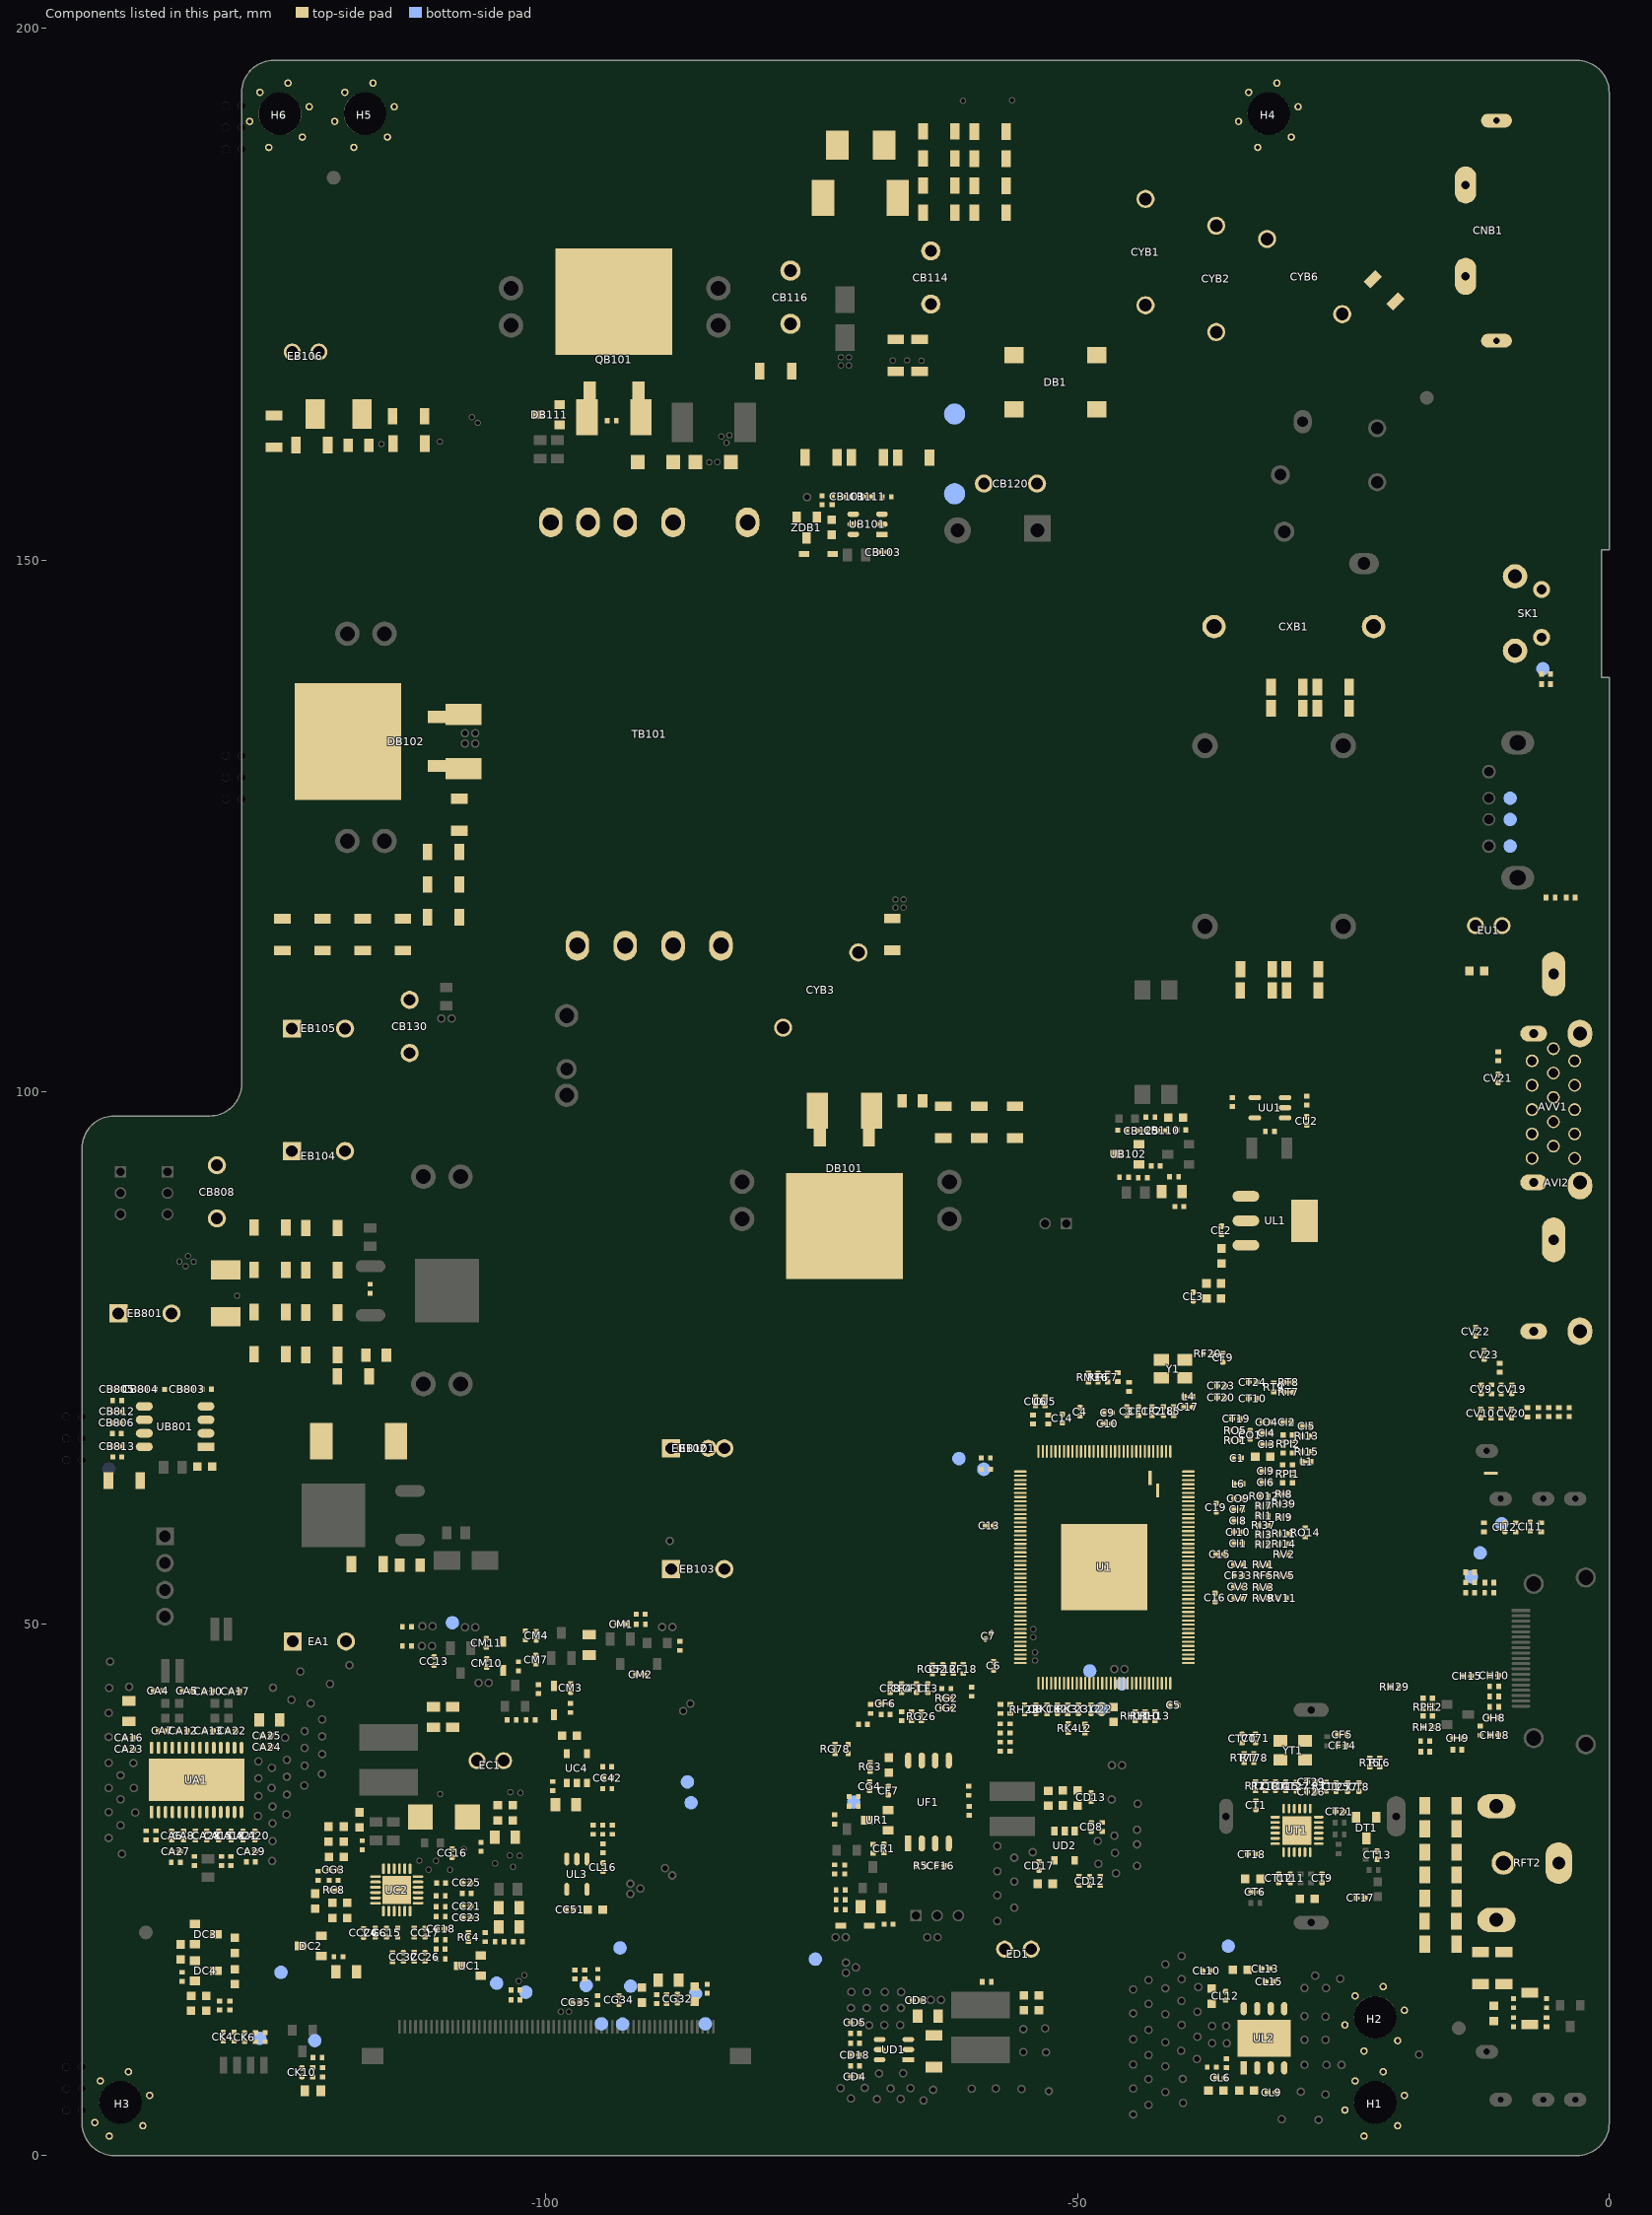
[diagram p0: the components of this part, seen from the top]
# Altium PCB MISC86383-9.PcbDoc (part 4 of 18)
Units mm, origin at the board's own origin, x right, y up, seen from the top; angles counter-clockwise.
Board outline 143.6 x 197 mm, 2 copper layers (TopLayer, BottomLayer), stack 1.571 mm thick; 743 components, 401 nets, 2996 pads, 1077 vias.
Unrouted connection lines stored in the file: 4.

## Components (designator, comment, footprint, x,y, rotation, side; value= is the part's Value field where it differs from the comment) (continued)
RH2 "Thick film resistor,RES,1/16W,0ohm,±1%,0402,SMD" R0402#1 -11.277,52.901 r0 top
RH10 "Thick film resistor,RES,1/16W,22ohm,±1%,0402,SMD" R0402#2 -43.635,41.317 r270 top
RH11 "Thick film resistor,RES,1/16W,22ohm,±1%,0402,SMD" R0402#2 -44.552,41.317 r270 top
RH13 "Thick film resistor,RES,1/16W,220ohm,±1%,0402,SMD" R0402#2 -42.714,41.317 r90 top
RH14 "Thick film resistor,RES,1/16W,1Kohm,±1%,0402,SMD" R0402#1 -12.142,39.947 r270 top
RH22 "Thick film resistor,RES,1/16W,100ohm,±1%,0402,SMD" R0402#2 -54.976,41.94 r90 top
RH28 "NC/10Kohm-0402-±5%-1/16W" R0402#2 -17.069,40.284 r0 top
RH29 "NC/15Kohm-0402-±1%-1/16W" R0402#2 -20.194,44.061 r0 top
RI1 "150ohm-0402-±1%-1/16W" R0402#2 -32.482,60.162 r180 top
RI2 "NC/150ohm-0402-±1%-1/16W" R0402#2 -32.482,57.483 r180 top
RI3 "NC/75ohm-0402-±5%-1/16W" R0402#2 -32.482,58.372 r0 top
RI7 "68ohm-0402-±5%-1/16W" R0402#2 -32.482,61.077 r0 top
RI8 "NC/" R0402SC -30.59,62.194 r0 top
RI9 "Thick film resistor,RES,1/16W,75ohm,±1%,0402,SMD" R0402#2 -30.577,60.023 r0 top
RI10 "NC/SHORT" GND -11.112,64.16 r0 top
RI11 "NC/0ohm-0402-±5%-1/16W" R0402#2 -30.577,58.486 r180 top
RI13 "NC/0ohm-0402-±5%-1/16W" R0402#2 -28.443,67.655 r180 top
RI14 "NC/0ohm-0402-±5%-1/16W" R0402#2 -30.566,57.495 r180 top
RI15 "NC/0ohm-0402-±5%-1/16W" R0402#2 -28.443,66.182 r180 top
RI37 "68ohm-0402-±5%-1/16W" R0402#2 -32.482,59.248 r0 top
RI39 "NC/75ohm-0402-±5%-1/16W" R0402#2 -30.577,61.28 r180 top
RK1 "NC/1K5ohm-0402-±5%-1/16W" R0402#1 -121.006,7.823 r90 top
RK3 "Thick film resistor,RES,1/16W,1Kohm,±1%,0402,SMD" R0402#2 -50.907,41.975 r270 top
RK4 "12Kohm-0402-±1%-1/16W" R0402#2 -50.874,40.187 r270 top
RK6 "1K2ohm-0402-±1%-1/16W" R0402#1 -5.944,139.294 r180 top
RK13 "Thick film resistor,RES,1/16W,22ohm,±1%,0402,SMD" R0402#1 -129.316,11.166 r270 top
RK15 "Thick film resistor,RES,1/16W,4.7Kohm,±1%,0402,SMD" R0402#1 -126.39,11.125 r270 top
RK16 "Thick film resistor,RES,1/16W,1Kohm,±1%,0402,SMD" R0402#1 -127.305,11.125 r270 top
RK18 "NC/33Kohm-0402-±5%-1/16W" R0402#2 -52.881,41.978 r270 top
RK20 "NC/10Kohm-0402-±5%-1/16W" R0402#1 -121.463,9.195 r0 top
RK21 "Thick film resistor,RES,1/16W,510ohm,±1%,0402,SMD" R0402#1 -121.92,7.823 r270 top
RL3 "NC/Thick film resistor,RES,1/16W,4.7Kohm,±5%,0402,SMD" R0402#1 -95.555,30.632 r270 top
RL4 "150ohm-0402-±1%-1/16W" R0402#1 -35.992,8.687 r270 top
RL5 "91ohm-0402-±1%-1/16W" R0402#1 -37.37,8.306 r180 top
RL7 "Thick film resistor,RES,1/16W,4.7Kohm,±1%,0402,SMD" R0402#1 -93.726,30.632 r270 top
RL50 "NC/10Kohm-0402-±5%-1/16W" R0402#1 -94.628,28.892 r90 top
RL51 "Thick film resistor,RES,1/16W,10Kohm,±1%,0402,SMD" R0402#1 -94.64,30.632 r270 top
RM1 "Thick film resistor,RES,1/16W,4.7Kohm,±1%,0402,SMD" R0402#1 -91.072,50.902 r180 top
RM2 "200Kohm-0402-±1%-1/16W" R0402#1 -91.059,49.962 r180 top
RM3 "Thick film resistor,RES,1/16W,10Kohm,±1%,0402,SMD" R0402#2 -48.969,73.156 r270 top
RM4 "Thick film resistor,RES,1/16W,4.7Kohm,±1%,0402,SMD" R0402#1 -87.376,47.917 r90 top
RM5 "Thick film resistor,RES,1/16W,4.7Kohm,±1%,0402,SMD" R0402#1 -97.665,42.083 r90 top
RM6 "NC/4K7ohm-0402-±5%-1/16W" R0402#1 -101.917,48.895 r270 top
RM7 "Thick film resistor,RES,1/16W,47Kohm,±1%,0402,SMD" R0402#1 -100.711,43.853 r90 top
RM8 "Thick film resistor,RES,1/16W,4.7Kohm,±1%,0402,SMD" R0402#1 -103.2,40.957 r180 top
RM10 "Thick film resistor,RES,1/16W,4.7Kohm,±1%,0402,SMD" R0402#1 -101.422,40.957 r0 top
RM12 "Thick film resistor,RES,1/16W,100Kohm,±1%,0402,SMD" R0402#1 -102.565,45.999 r90 top
RO1 "Thick film resistor,RES,1/16W,510ohm,±1%,0402,SMD" R0402#2 -35.174,67.262 r0 top
RO2 "NC/100ohm-1206-±5%-1/4W" R1206 -7.468,13.813 r90 top
RO5 "Thick film resistor,RES,1/16W,510ohm,±1%,0402,SMD" R0402#2 -35.174,68.189 r0 top
RO6 "NC/10Kohm-0402-±5%-1/16W" R0402#1 -8.992,14.321 r270 top
RO9 "NC/100ohm-0402-±5%-1/16W" R0402#1 -8.992,12.543 r90 top
RO10 "NC/1Kohm-0402-±5%-1/16W" R0402#1 -5.893,14.321 r270 top
RO12 "Thick film resistor,RES,1/16W,75ohm,±1%,0402,SMD" R0402#2 -32.482,61.991 r180 top
RO14 "Thick film resistor,RES,1/16W,0ohm,±1%,0402,SMD" R0402#2 -28.596,58.575 r90 top
RPH2 "Resistor array,RES ARRAY,1/16W,4×10Kohm,±5%,0402,SMD" RA0402 -17.056,42.164 r180 top
RPI1 "Resistor array,RES ARRAY,1/16W,4×10Kohm,±5%,0402,SMD" RA0402 -30.247,64.099 r0 top
RPI2 "NC/Resistor array,RES ARRAY,1/16W,4×10Kohm,±5%,0402,SMD" RA0402 -30.221,66.906 r0 top
RR1 "NC/1Kohm-0402-±5%-1/16W" R0402#1 -71.044,32.842 r180 top
RR2 "NC/100Kohm-0402-±5%-1/16W" R0402#1 -71.044,33.757 r0 top
RR5 "NC/0ohm-0402-±5%-1/16W" R0402#1 -69.207,28.84 r270 top
RR6 "NC/0ohm-0402-±5%-1/16W" R0402#1 -72.847,31.598 r270 top
RT2 "Thick film resistor,RES,1/16W,100ohm,±1%,0402,SMD" R0402#2 -33.258,34.736 r90 top
RT5 "Thick film resistor,RES,1/16W,33ohm,±1%,0402,SMD" R0402#2 -22.496,36.946 r90 top
RT6 "Thick film resistor,RES,1/16W,33ohm,±1%,0402,SMD" R0402#2 -21.581,36.946 r90 top
RT7 "NC/" R0402SC -30.163,71.794 r180 top
RT8 "NC/" R0402SC -30.163,72.721 r180 top
RT9 "NC/430ohm-0402-±5%-1/16W" R0402#2 -31.534,72.238 r90 top
RT11 "Thick film resistor,RES,1/16W,1.8Kohm,±1%,0402,SMD" R0402#2 -26.642,34.698 r270 top
RT18 "Thick film resistor,RES,1/16W,10Kohm,±1%,0402,SMD" R0402#2 -32.344,34.724 r90 top
RT77 "NC/" R0402SC -34.337,37.384 r90 top
RT78 "NC/" R0402SC -33.419,37.384 r90 top
RU4 "NC/Thick film resistor,RES,1/16W,4.7Kohm,±1%,0402,SMD" R0402#1 -35.433,99.06 r270 top
RU45 "NC/Thick film resistor,RES,1/16W,5.6Kohm,±1%,0402,SMD" R0402#1 -28.448,99.187 r90 top
RV1 "NC/33ohm-0402-±5%-1/16W" R0402#2 -32.494,55.578 r0 top
RV2 "NC/75ohm-0402-±5%-1/16W" R0402#2 -30.561,56.512 r180 top
RV3 "NC/33ohm-0402-±5%-1/16W" R0402#2 -32.494,53.444 r0 top
RV4 "NC/10Kohm-0402-±5%-1/16W" R0402#1 -10.153,72.056 r270 top
RV5 "NC/75ohm-0402-±5%-1/16W" R0402#2 -30.564,54.562 r180 top
RV6 "NC/100ohm-0402-±5%-1/16W" R0402#1 -11.067,72.056 r270 top
RV9 "NC/33ohm-0402-±5%-1/16W" R0402#2 -32.494,52.428 r0 top
RV10 "NC/100ohm-0402-±5%-1/16W" R0402#1 -11.119,69.775 r270 top
RV11 "NC/75ohm-0402-±5%-1/16W" R0402#2 -30.767,52.428 r180 top
RV12 "Thick film resistor,RES,1/16W,4.7Kohm,±1%,0402,SMD" R0402#1 -56.35,38.456 r270 top
RV13 "Thick film resistor,RES,1/16W,4.7Kohm,±1%,0402,SMD" R0402#1 -57.277,38.456 r270 top
RV14 "NC/10Kohm-0402-±5%-1/16W" R0402#1 -10.205,69.775 r270 top
RV18 "Thick film resistor,RES,1/16W,100ohm,±1%,0402,SMD" R0402#1 -57.262,40.162 r270 top
RV19 "Thick film resistor,RES,1/16W,100ohm,±1%,0402,SMD" R0402#1 -56.348,40.162 r270 top
RV20 "Thick film resistor,RES,1/16W,0ohm,±1%,0402,SMD" R0402#1 -60.198,32.41 r90 top
RV21 "Thick film resistor,RES,1/16W,0ohm,±1%,0402,SMD" R0402#1 -60.223,34.29 r90 top
RV22 "NC/Thick film resistor,RES,1/16W,0ohm,±1%,0402,SMD" R0402#1 -5.69,69.901 r90 top
RV23 "NC/Thick film resistor,RES,1/16W,0ohm,±1%,0402,SMD" R0402#1 -3.759,69.901 r90 top
S/N1 "Barcode" Barcode -33.114,77.987 r180 bottom
S/N2 "Barcode" Barcode -70.231,43.434 r180 bottom
SK1 "Tact switch,Tact Switch,160±50gf,7.0×10.3×7.0mm,DIP,106520070,VAST" KEY-HD-6 -3.85,145 r90 top locked
STV "TEST" TP -86.677,35.128 r180 bottom
TB101 "Transformer,Transformer,EQ2612,230uH,0.2×2P,25Ts,H14.5MAX,SYEQ2613-T012017A(BLACK),DIP,SQ" T/EQ2612*10 -90.278,131.267 r270 top locked
TP "TEST" TP -92.786,12.357 r180 bottom
TP-TDT "NC/" TP-TDT -61.557,160.007 r270 bottom
TVCOM "TEST" TP -96.202,15.989 r180 bottom
U1 "TV main chip,IC Main Chip,TSU69KBPT-003D,32bit,Signal-Core,S2EPLQFP156,SMD,Mstar" QFP156/0.4-2 -47.471,55.313 r90 top locked
UA1 "Audio amplifier IC,Class D,2×10W@13V@8ohm,HTSSOP-28,SMD,CS3817BEO,HRXK" SSOP28/0.65-5 -132.845,35.316 r90 top
UART_RX "TEST" TP -12.135,56.667 r90 bottom
UART_TX "TEST" TP -12.954,54.419 r90 bottom
UB101 "PWM controller,IC PWM Controller,100KHZ,SOT23-6,SMD,LD5537B3GL,Leadtrend" SOT-26 -69.736,153.391 r270 top
UB101及周围贴片器件 "NC/Conformal coating,25kg/Can,Peters" PCB_TIME 33.85,168.811 r90 top
UB102 "Regulator IC,IC Regulator,2.50V,0.4%,SOT-23,SMD,BR431M-A,Blue Rocket" SOT-23-RAK -45.237,94.158 r90 top
UB801 "PWM controller,IC PWM Controller,120KHz,SOP-8,SMD,AL3353S-13,DIODES" SO-8A -134.861,68.545 r180 top
UB801及周围贴片器件 "NC/Conformal coating,25kg/Can,Peters" PCB_TIME 34.15,168.811 r90 top
UC1 "Regulator IC,IC Regulator,2.50V,0.4%,SOT-23,SMD,BR431M-A,Blue Rocket" SO-23-1 -107.137,17.843 r90 top
UC2 "Tcon driver IC,IC Tcon  Driver,VQFN-24L,SMD,ANX6732AAQX,ANAX" QFN24/0.5-5 -114.014,24.973 r0 top
UC4 "Operational amplifier,AMP,1,9MHz,SOT-23-5,SMD,SGM8425AYN5G/TR,SGMICRO" SOT-23-5 -97.079,36.411 r0 top
UD1 "DC-DC IC,IC DC-DC,Syn,2A,18V,600KHz,SOT23-6,SMD,TMI3252T,TOLL" TSOT23-6 -67.259,9.957 r180 top
UD2 "DC-DC IC,IC DCDC,Syn,1.2A,6.0V,1.5MHz,SOT23-5,SMD,TMI3408,TOLL" SOT-23-5 -51.199,29.132 r180 top
UF1 "SPI flash IC,IC SPI FLASH,4MB,32Mb,SOIC8,SMD,W25Q32JVSSIQ,Winbond" SOIC8 -64.011,33.242 r90 top
UL1 "LDO IC,IC LDO,1A,1.8V,15V,SOT-223,SMD,SCJT1117B-1.8V,CJKJ" SOT-223 -31.413,87.898 r270 top
UL2 "LDO IC,IC LDO,1A,3.3V+ADJ,12V,ESOP-8,SMD,LC1118CS8TRAD33,Leadchip" SOP8/1.27-3 -32.461,11.024 r90 top
UL3 "LDO IC,IC LDO,0.3A,3.3V,6V,SOT23-5,SMD,LC1463CB5ATR33,Leadchip" SOP23-5-1 -97.079,26.454 r180 top
UR1 "NC/SGM810-SXN3L" SO-23-1 -68.826,31.533 r90 top
USB0_DM "TEST" TP -9.31,125.63 r180 bottom
USB0_DP "TEST" TP -9.31,127.63 r180 bottom
USB_5V "TEST" TP -9.31,123.13 r180 bottom
UT1 "Silicon tuner IC,IC Si Tuner,QFN24,SMD,R842,Rafael" QFN24/0.5-3 -29.36,30.57 r180 top
UU1 "NC/Current limit switch,IC OCP,0.4-2A adj,5.5V,H,SOT23-5,SMD,SY6280AAAC,SILERGY" SOP23-5-1 -31.902,98.527 r90 top
VCC_DDR "TEST" TP -48.844,45.568 r90 bottom
VCC_PANEL "TEST" TP -108.788,50.102 r0 bottom
VMID/SCL "TEST" TP -58.814,64.529 r180 bottom
VMID/SDA "TEST" TP -61.15,65.532 r90 bottom
VOFF "TEST" TP -104.623,16.205 r180 bottom
VON "TEST" TP -124.904,17.221 r180 bottom
XAO "TEST" TP -85.915,15.202 r180 bottom
XCM101B1-PT "PCB_NAME" PCB_NAME -76.708,16.002 r180 top
XXXXXX "PCB_TIME" PCB_TIME -85.471,23.495 r0 top
XXXXXXXXXXXXXXX "PCB_NAME" PCB_NAME -80.137,19.939 r180 top
Y1 "Passive crystal oscillator,SPXO,24MHz,±10ppm,12pF,SMD3225,SMD,SX32Y024000BC1T-Z,TKD" XTAL-S-3 -41.006,73.97 r180 top
YT1 "NC/Passive standard-package crystal oscillator,SPXO,24MHz,±20ppm,16pF,3.2×2.5,SMD,SMD3225 24.000MHZ,JWT" XTAL-S-10 -29.758,38.102 r0 top
ZDB1 "NC/BZX84C24(BLUE ROCKET)" SO-23 -75.463,153.06 r0 top
用于U1上 "Glue,0.1g,silicone,ZJ" "Heat-Shrinkable Tube" 1.429,25.711 r90 top

## Footprints (in the part's own frame and the unit in brackets; to place one, negate y for a bottom-side part, rotate by r counter-clockwise, add the part's x,y. Pads: shape width x height; smd on the part's side, far side on the other; paste and mask are expansions set on the pad)
AI_GRIPPER_V [mm] "3D shape for vertical type AI equipment"
  round 1.5 on Mech5: 0(0,-2.5) 1(0,0) 2(0,2.5)
  body extent -29.13,-4.7 2.5,4.7, height 54.74
ANT-IEC14.5-H-4 [mm] "联宏达；13.2×12.4×7.7mm LHD-020 中心高度6.3mm 160323(18.03.09更新脚距）,向内扩宽丝印,0703_2018（18.08.29 更新短槽?"
  oval 2.5x3.8 on Top Overlay paste-4 mask-4: 0(-5.35,6.1) 0(5.35,6.1)
  round 2.4 on Top Overlay: 0(0,5.45)
  oval 4.1x2.7 on Top Overlay paste-4 mask-4: 0(0,0.25)
  round 2.2 hole 1.4: 1(0,5.45)
  oval 2.3x3.6 hole 1.3 slot 2.6 at 90 deg: 2(-5.35,6.1) 4(5.35,6.1)
  oval 3.9x2.5 hole 1.2 slot 2.6 at 0 deg: 3(0,0.25)
  KeepOutLayer pour cut-out: 0,3.95 -0.574,4.064 -1.061,4.389 -1.386,4.876 -1.5,5.45 -1.5,5.45 -1.386,6.024 -1.061,6.511 -0.574,6.836 0,6.95 0,6.95 0.574,6.836 1.061,6.511 1.386,6.024 1.5,5.45 1.5,5.45 1.386,4.876 1.061,4.389 0.574,4.064 0,3.95
  silkscreen extent -6.3,0 6.3,7.9, body extent -7.55,-35.2 7.55,7.7, height 13.76
ASSE4.0C-3#1 [mm] "定位孔(顶底层上锡)(17.12.09更新过孔位置）18.11.22 更新paste形状为扇形。"
  round 4 hole 4 unplated mask+0: 0(0,0)
  round 0.7 hole 0.4: 1(-2.85,-0.725) 2(-1.893,2.011) 3(0.75,2.875) 4(2.75,0.65) 5(2.105,-2.203) 6(-1.05,-3.175)
  KeepOutLayer pour cut-out: 0,-2.3 -0.88,-2.125 -1.626,-1.626 -2.125,-0.88 -2.3,0 -2.3,0 -2.125,0.88 -1.626,1.626 -0.88,2.125 0,2.3 0,2.3 0.88,2.125 1.626,1.626 2.125,0.88 2.3,0 2.3,0 2.125,-0.88 1.626,-1.626 0.88,-2.125 0,-2.3
ASSE4.0C-3#2 [mm] "定位孔(顶底层上锡)(17.12.09更新过孔位置）18.11.22 更新paste形状为扇形。"
  round 4 hole 4 unplated mask+0: 0(0,0)
  round 0.7 hole 0.4: 1(-2.412,-1.894) 2(-1.893,2.011) 3(0.75,2.875) 4(2.75,0.65) 5(2.105,-2.203) 6(-1.05,-3.175)
  KeepOutLayer pour cut-out: 0,-2.3 -0.88,-2.125 -1.626,-1.626 -2.125,-0.88 -2.3,0 -2.3,0 -2.125,0.88 -1.626,1.626 -0.88,2.125 0,2.3 0,2.3 0.88,2.125 1.626,1.626 2.125,0.88 2.3,0 2.3,0 2.125,-0.88 1.626,-1.626 0.88,-2.125 0,-2.3
AV3-H14-15 [mm] "宇球；RC075-F03L3BY-A; 中心高度：5.5mm;15.11.24;170401兼容物料，更新高度;170802加大接地脚焊盘（18.03.09更新孔距）"
  oval 2.8x2.5 on Top Overlay: 0(-14,2.75) 0(0,2.75) 0(14,2.75)
  oval 1.7x2.7 on Top Overlay: 0(-14,7.1) 0(0,7.1) 0(14,7.1)
  oval 1.5x2.5 hole 0.8 slot 1.8 at 90 deg: 1(-14,7.1) 3(0,7.1) 5(14,7.1)
  oval 2.6x2.3 hole 1.3 slot 1.6 at 0 deg: 2(-14,2.75) 6(14,2.75)
  oval 2.6x2.3 hole 1.3 slot 1.6 at 0 deg copper offset -0.3,0: 4(0,2.75)
  silkscreen extent -20.3,0 20.3,7.8, body extent -20.1,-9 20.1,7.9, height 10.7
B/YBS3010A [mm] "YJ,YBS3010A,18.04.17"
  rect 1.5x1.8 smd: 1(2.55,3.9) 2(2.55,-3.9) 3(-2.55,-3.9) 4(-2.55,3.9)
  silkscreen extent -3.35,-3.7 3.35,5.73, body extent -3.35,-3.7 3.35,3.7, height 1.5
Barcode [mm]
  round 0.3 on Mech2: 0(0,0)
  silkscreen extent -15,-4 15,4
C0402 [mm] "片式电容  2018.10.7 替换为兼容0201封装"
  rrect50% 0.45x0.5 smd mask+0.051: 1(-0.425,0) 2(0.425,0)
  rect 0.3x0.3 smd mask+0.051: 1(-0.25,0) 2(0.25,0)
  rect 0.6x0.6 on Top Solder: 2(0,0)
  TopLayer pour cut-out: -0.318,0.302 -0.318,-0.303 0.306,-0.303 0.306,0.302
  silkscreen extent -0.87,-0.47 0.87,0.47, body extent -0.5,-0.25 0.5,0.25, height 0.5
C0603 [mm] "片式电容"
  rect 0.8x0.8 smd mask+0.076: 1(-0.706,0) 2(0.706,0)
  silkscreen extent -1.39,-0.62 1.39,0.62, body extent -0.8,-0.4 0.8,0.4, height 0.8
C0805 [mm] "片式电容"
  rect 0.9x1.25 smd mask+0.076: 1(-0.966,0) 2(0.966,0)
  silkscreen extent -1.73,-0.84 1.73,0.84, body extent -1,-0.62 1,0.63, height 1.25
C1206 [mm] "片式电容"
  rect 1x1.6 smd mask+0.076: 1(-1.5,0) 2(1.5,0)
  silkscreen extent -2.39,-1.02 2.39,1.02, body extent -1.6,-0.8 1.6,0.8, height 1.3
CAP6.5*5-V-5-1 [mm] "TDK，CC45SL3DD680JYSNA，外K型引脚，AI，0713_2018"
  round 2.1 on Top Overlay: 0(-2.5,0) 0(2.5,0)
  round 1.9 hole 1.2 mask+0.051: 1(-2.5,0) 2(2.5,0)
  BottomLayer lines w0.6: -2.19,0.39 -2.238,0.42 -4.056,1.556 ; 2.89,0.31 2.92,0.262 2.92,0.262 4.056,-1.556 ; -2.5,0 -4.056,1.556 ; 2.5,0 4.056,-1.556 ; -2.89,-0.31 -2.92,-0.262 -4.056,1.556 ; 2.19,-0.39 2.238,-0.42 4.056,-1.556
  silkscreen extent -5.5,-2.5 5.5,2.5
CAP8*2.5-V-5 [mm] "C242G472J20A201(编带/法拉)"
  round 1.8 hole 1.1: 1(-2.5,0) 2(2.5,0)
  round 2 on Top Overlay: 1(-2.5,0) 1(2.5,0)
  BottomLayer lines w0.6: -2.15,0.456 -2.215,0.493 -2.5,0.657 -2.602,0.717 -4.056,1.556 ; 2.956,0.35 4.056,-1.556 ; -2.5,0 -2.652,0.152 -2.986,0.486 -4.056,1.556 ; 2.5,0 4.056,-1.556 ; -2.956,-0.35 -2.993,-0.285 -3.157,0 -3.434,0.479 -4.056,1.556 ; 2.15,-0.456 4.056,-1.556
  silkscreen extent -4,-1.25 4,1.25
CAP9.8*4-V-5 [mm] "SHM;DCH472M36Y5UN6FL5A0;15.09.06"
  round 1.7 hole 1.1: 1(-2.5,0) 2(2.5,0)
  round 1.9 on Top Overlay: 3(-2.5,0) 4(2.5,0)
  BottomLayer lines w0.6: 2.19,-0.39 2.238,-0.42 ; -2.89,-0.31 -2.92,-0.262 ; 2.5,0 4.056,-1.556 ; -2.5,0 -4.056,1.556 ; 2.89,0.31 2.92,0.262 ; -2.19,0.39 -2.238,0.42 ; 4.056,-1.556 3.084,0 2.92,0.262 ; 4.056,-1.556 2.238,-0.42 ; 2.238,-0.42 2.238,-0.42 ; 2.238,-0.42 2.238,-0.42 ; -2.92,-0.262 -4.056,1.556 ; -2.92,-0.262 -2.92,-0.262 ; -2.92,-0.262 -2.92,-0.262 ; 2.92,0.262 2.92,0.262 ; 2.92,0.262 2.92,0.262 ; -2.238,0.42 -4.056,1.556 ; -2.238,0.42 -2.238,0.42 ; -2.238,0.42 -2.238,0.42
  silkscreen extent -4.91,-2 4.9,2, body extent -5.49,-2.5 5.5,2.5, height 12.5
CAP10*4.5-V-5#1 [mm] "YU102472M090DAND5H，陶瓷电容，17.12.22"
  round 1.7 hole 1.1: 1(-2.5,0) 2(2.5,0)
  round 1.9 on Top Overlay: 41(2.5,0) 42(-2.5,0)
  BottomLayer lines w0.6: -2.89,-0.31 -2.92,-0.262 -4.056,1.556 ; -2.5,0 -4.056,1.556 ; -2.19,0.39 -2.238,0.42 -4.056,1.556 ; 2.19,-0.39 2.238,-0.42 2.5,-0.584 2.923,-0.848 4.056,-1.556 ; 2.5,0 4.056,-1.556 ; 2.89,0.31 2.92,0.262 ; 2.92,0.262 4.056,-1.556
  silkscreen extent -5.55,-2.25 5.55,2.25
CAP10*4.5-V-5#2 [mm] "YU102472M090DAND5H，陶瓷电容，17.12.22"
  round 1.7 hole 1.1: 1(-2.5,0) 2(2.5,0)
  round 1.9 on Top Overlay: 41(2.5,0) 42(-2.5,0)
  BottomLayer lines w0.6: -2.19,0.39 -2.238,0.42 -4.056,1.556 ; 2.89,0.31 2.92,0.262 3.084,0 4.056,-1.556 ; -2.5,0 -4.056,1.556 ; 2.5,0 4.056,-1.556 ; -2.89,-0.31 -2.92,-0.262 -4.056,1.556 ; 2.19,-0.39 2.238,-0.42 4.056,-1.556
  silkscreen extent -5.55,-2.25 5.55,2.25
CAP13*5-V-10-1 [mm] "Walsin;YU1AH471M060DAMD0H;160718（18.03.15  更新孔径）"
  round 1.7 hole 1.2: 1(-5,0) 2(5,0)
  round 1.9 on Top Overlay: 61(-5,0) 61(5,0)
  silkscreen extent -5.71,-3 5.81,3
CAP18*8.5-V-15 [mm] "PX334K3ID49H200D9R(凯励)(18.01.12更新孔径）(18.07.18 更新丝印框，加了公差）(09/29/2019添加白油块)"
  round 2.2 hole 1.4: 1(-7.5,0) 2(7.5,0)
  round 2.4 on Top Overlay: 77(7.5,0) 78(-7.5,0)
  silkscreen extent -9.28,-4.45 9.28,4.45, body extent -9.25,-4.45 9.25,4.45, height 14.5
CAUTION [mm]
  silkscreen extent -10.17,-3.72 12.33,4.08
COLD [mm]
CON2-H8.6-1 [mm] "输入插座（ST-A03-005DT8+M02）东莞阳琦电子;15.01.21"
  round 3.3 on Keep-Out: 0(-6.5,-4.7) 0(6.5,-4.7)
  oval 1.5x3.1 on Top Overlay: 1(-10.35,-3.4) 1(10.35,-3.4)
  oval 3.5x2 hole 0.8 slot 2.2 at 0 deg: 1(-4.3,-0.5) 2(4.3,-0.5)
  oval 3.7x2.2 on Top Overlay: 1(-4.3,-0.5) 1(4.3,-0.5)
  oval 1.3x2.9 hole 0.6 slot 2.2 at 90 deg: 3(10.35,-3.4) 4(-10.35,-3.4)
  silkscreen extent -11,-14 11,0, body extent -11.02,-14 10.98,0, height 12.73
CQC [mm]
D2PAK3 [mm] "伟达电子；SFS1006G;增加TO-252兼容；160309"
  oval 2.794x1.143 smd: 1(5.542,-2.2) 3(5.542,2.4)
  rect 2.794x1.143 smd: 1(5.544,-2.2) 3(5.544,2.4)
  rect 3.4x2 smd paste-5 mask-5: 1(7.494,-2.44) 3(7.494,2.64)
  rect 10x11 smd paste-11 mask-11: 2(-3.356,0.1)
  rect 6x6 smd paste-10 mask-11: 2(-2.158,0.1)
  TopLayer pour cut-out: 3.373,2.4 6.497,2.4 6.497,-2.245 6.438,-2.54 6.271,-2.791 6.02,-2.958 5.725,-3.017 5.725,-3.017 5.725,-2.199 4.141,-2.199 4.141,-3.024 3.847,-2.966 3.598,-2.799 3.432,-2.55 3.373,-2.256 3.373,-2.256
  silkscreen extent -9.13,-5.69 4.84,5.89, body extent -6.91,-5.15 8.79,5.35, height 4.7
DB15-HF-1 [mm] "兴万联电子：WLHD-051A"
  oval 4.4x2.4 on Top Overlay: 0(-12.5,5.227) 0(12.5,5.227)
  round 1.2 hole 0.9: 1(4.33,7.247) 2(2.04,7.247) 3(-0.25,7.247) 4(-2.54,7.247) 5(-4.83,7.247) 6(5.475,5.247) 7(3.185,5.247) 8(0.895,5.247) 9(-1.395,5.247) 10(-3.685,5.247) 11(4.33,3.247) 12(2.04,3.247) 13(-0.25,3.247) 14(-2.54,3.247) 15(-4.83,3.247)
  oval 4.2x2.2 hole 1 slot 3 at 0 deg: 16(-12.5,5.227) 17(12.5,5.227)
  round 1.5 on Top Overlay: 30(-4.83,3.247) 31(-2.54,3.247) 32(-0.25,3.247) 33(2.04,3.247) 34(4.33,3.247) 35(5.475,5.247) 36(3.185,5.247) 37(0.895,5.247) 38(-1.395,5.247) 39(-3.685,5.247) 40(-4.83,7.247) 41(-2.54,7.247) 42(-0.25,7.247) 43(2.04,7.247) 44(4.33,7.247)
  BottomLayer pour cut-out: -4.814,8.609 -4.814,5.885 -4.587,5.885 -4.443,5.742 -3.456,5.742 -3.175,5.461 -3.175,5.029 -3.454,4.75 -4.42,4.75 -4.56,4.609 -4.797,4.609 -4.83,4.576 -4.83,1.885 4.33,1.885 4.33,3.247 4.298,3.279 4.298,4.609 4.105,4.609 3.95,4.764 2.44,4.764 2.285,4.609 1.817,4.609 1.664,4.763 0.648,4.763 0.368,5.042 0.368,5.474 0.622,5.728 1.651,5.728 1.803,5.88 2.286,5.88 2.438,5.728 3.95,5.728 4.107,5.885 4.33,5.885 4.33,8.609
  silkscreen extent -15.59,0 15.59,9.48, body extent -16.75,-62.85 16.75,8.75, height 14.13
DIODE-S0402 [mm] "DVD上使用的ESD"
  rect 0.45x0.55 smd mask+0.051: A(-0.425,0) K(0.425,0)
  silkscreen extent -0.8,-0.43 0.91,0.43, body extent -0.5,-0.25 0.5,0.25, height 0.5
DIODE-S0603 [mil]
  rect 32x40 smd: A(-29.5,0) K(29.5,0)
  silkscreen extent -55,-30 63,30, body extent -31,-16 31,16, height 31
DIODE-S-1 [mm] "SK34(18.09.07 去除0805电阻兼容）"
  rect 2.33x2.4 smd: A(-2.21,0) K(2.21,0)
  silkscreen extent -3.8,-1.4 4.04,1.4, body extent -2.63,-1.12 2.37,1.12, height 2
DIODE-S-2 [mm] "1N5819-SMA;170509去除兼容,20180607减少内距0.4mm以兼容SMAF"
  rect 1.8x2.8 smd: A(-2.2,0) K(2.2,0)
  silkscreen extent -3.5,-1.6 3.7,1.61, body extent -2.6,-1.4 2.6,1.4, height 1.91
DIODE-S-12 [mm] "Formosa MS ;BAV19WS THRU BAV21WS/PMEG2010BEA(高度为1.1mm)"
  rect 1x0.55 smd: A(1.35,0) K(-1.35,0)
  silkscreen extent -0.9,-0.67 0.9,0.67, body extent -1.35,-0.63 1.35,0.63, height 1
DIODE-S-14 [mm] "ROHM;FSL14"
  rect 1.3x1.35 smd: A(1.675,0) K(-1.675,0)
  silkscreen extent -1.55,-1 1.55,1, body extent -1.95,-1 1.95,1, height 1.08
DIODE-SMB [mm] "SMB或DO-214AA(MUR360(ON));14.05.28修改"
  rect 2.159x2.743 smd: A(2.2,0) K(-2.2,0)
  silkscreen extent -3.84,-2.24 3.84,2.24
DIODE-SMC [mm] "SM320C~SM3200;DO-214AB;14-03-07"
  rect 2.1x3.4 smd: A(3.505,0) K(-3.505,0)
  silkscreen extent -3.55,-3.11 3.55,3.92, body extent -4.07,-3.11 4.07,3.11, height 2.62
DOLBY_AS2 [mm] "杜比认证预留框，两行印刷，规格35.0*5.4mm"
EC(5*11)-V-2.5 [mm] "机插2.5间距"
  round 1.8 on Top Overlay: 0(-1.25,0) 0(1.25,0)
  round 0.5 on Keep-Out: 0(0,-0.787)
  round 1.6 hole 1.1: 1(-1.25,0) 2(1.25,0)
  BottomLayer lines w0.6: -1.64,-0.31 -1.67,-0.262 -2.806,1.556 ; -1.25,0 -2.806,1.556 ; -0.94,0.39 -0.988,0.42 -2.806,1.556 ; 0.94,-0.39 0.988,-0.42 2.806,-1.556 ; 1.25,0 2.806,-1.556 ; 1.64,0.31 1.67,0.262 ; 1.67,0.262 2.806,-1.556
  silkscreen extent -2.75,-2.75 3,2.75, body extent -2.48,-2.52 2.5,2.47, height 12.5
EC(6.3*11)-V-2.5#1 [mm] "机插2.5间距"
  round 0.5 on Keep-Out: 0(0,-0.889)
  round 1.6 hole 1.1: 1(-1.25,0) 2(1.25,0)
  round 1.8 on Top Overlay: 5(1.25,0) 6(-1.25,0)
  BottomLayer lines w0.6: -1.665,-0.275 -1.691,-0.225 ; -1.25,0 -2.664,1.685 ; -0.907,0.361 -0.952,0.395 ; 0.907,-0.361 0.952,-0.395 ; 1.25,0 2.664,-1.685 ; 1.665,0.275 1.691,0.225 ; -2.664,1.685 -1.691,-0.225 ; -2.664,1.685 -0.952,0.395 ; -1.691,-0.225 -1.691,-0.225 ; -1.691,-0.225 -1.691,-0.225 ; -0.952,0.395 -0.952,0.395 ; -0.952,0.395 -0.952,0.395 ; -0.952,0.395 -0.952,0.395 ; -0.952,0.395 -0.952,0.395 ; -0.952,0.395 -0.952,0.395 ; 0.952,-0.395 2.664,-1.685 ; 0.952,-0.395 0.952,-0.395 ; 0.952,-0.395 0.952,-0.395 ; 0.952,-0.395 0.952,-0.395 ; 0.952,-0.395 0.952,-0.395 ; 1.691,0.225 2.664,-1.685 ; 1.691,0.225 1.691,0.225
  silkscreen extent -3.17,-3.17 3.51,3.17, body extent -3,-3 2.98,2.99, height 12.5
EC(6.3*11)-V-2.5#2 [mm] "机插2.5间距"
  round 0.5 on Keep-Out: 0(0,-0.889)
  round 1.6 hole 1.1: 1(-1.25,0) 2(1.25,0)
  round 1.8 on Top Overlay: 5(1.25,0) 6(-1.25,0)
  BottomLayer lines w0.6: -1.665,-0.275 -1.691,-0.225 ; -1.25,0 -2.664,1.685 ; -0.907,0.361 -0.952,0.395 ; 0.907,-0.361 0.952,-0.395 ; 1.25,0 2.664,-1.685 ; 1.665,0.275 1.691,0.225 2.664,-1.685 ; -2.664,1.685 -1.691,-0.225 ; -2.664,1.685 -0.952,0.395 ; -1.691,-0.225 -1.691,-0.225 ; -0.952,0.395 -0.952,0.395 ; -0.952,0.395 -0.952,0.395 ; -0.952,0.395 -0.952,0.395 ; -0.952,0.395 -0.952,0.395 ; 0.952,-0.395 0.952,-0.395 ; 0.952,-0.395 1.25,-0.62 2.664,-1.685 ; 0.952,-0.395 0.952,-0.395
  silkscreen extent -3.17,-3.17 3.51,3.17, body extent -3,-3 2.98,2.99, height 12.5
EC(6.3*11)-V-2.5#3 [mm] "机插2.5间距"
  round 0.5 on Keep-Out: 0(0,-0.889)
  round 1.6 hole 1.1: 1(-1.25,0) 2(1.25,0)
  round 1.8 on Top Overlay: 5(1.25,0) 6(-1.25,0)
  BottomLayer lines w0.6: -1.665,-0.275 -1.691,-0.225 -2.664,1.685 ; -1.25,0 -2.664,1.685 ; -0.907,0.361 -0.952,0.395 -2.664,1.685 ; 0.907,-0.361 2.664,-1.685 ; 1.25,0 2.664,-1.685 ; 1.665,0.275 2.664,-1.685
  silkscreen extent -3.17,-3.17 3.51,3.17, body extent -3,-3 2.98,2.99, height 12.5
EC(8*11)-V-3.5 [mm]
  rect 1.6x1.6 hole 1: 1(-1.75,0)
  rect 1.8x1.8 on Top Overlay: 1(-1.75,0)
  round 1.8 on Top Overlay: 1(1.75,0)
  round 1.6 hole 1: 2(1.75,0)
  silkscreen extent -4.25,-4.25 4.45,4.25, body extent -3.98,-3.98 4.01,4.01, height 12.51
EC(10*12.5)-V-5#1 [mm] "机插5间距"
  round 0.5 on Keep-Out: 0(-0.75,0)
  rect 1.7x1.7 hole 1.1: 1(-2.5,0)
  rect 1.9x1.9 on Top Overlay: 1(-2.5,0)
  round 1.9 on Top Overlay: 1(2.5,0)
  round 1.7 hole 1.1: 2(2.5,0)
  BottomLayer lines w0.6: -2.89,-0.31 -2.92,-0.262 ; -2.5,0 -4.056,1.556 ; -2.19,0.39 -2.238,0.42 ; 2.19,-0.39 2.238,-0.42 ; 2.5,0 4.056,-1.556 ; 2.89,0.31 2.92,0.262 2.92,0.262 ; -4.056,1.556 -2.92,-0.262 ; -4.056,1.556 -2.238,0.42 ; -2.92,-0.262 -2.92,-0.262 ; -2.92,-0.262 -2.92,-0.262 ; -2.238,0.42 -2.238,0.42 ; -2.238,0.42 -2.238,0.42 ; 2.238,-0.42 2.238,-0.42 ; 2.238,-0.42 2.238,-0.42 ; 2.238,-0.42 4.056,-1.556 ; 2.92,0.262 2.92,0.262 ; 2.92,0.262 4.056,-1.556
  silkscreen extent -5.2,-5.21 5.57,5.21, body extent -4.98,-4.99 5.01,4.99, height 14.01